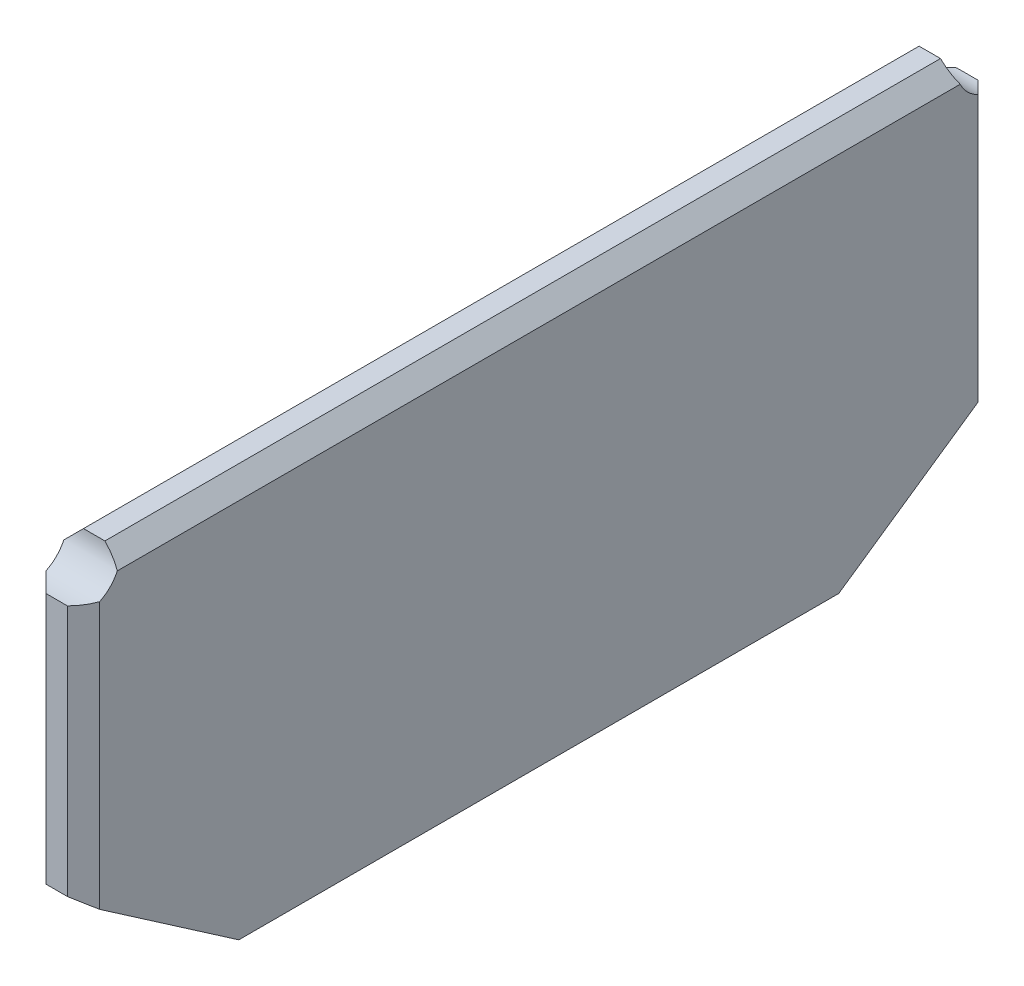
SolidWorks part; units mm, degrees
material "Q235-A"
ref_plane "Front Plane" through (0, 0, 0) normal (0, 0, 1) x (1, 0, 0)
ref_plane "Top Plane" through (0, 0, 0) normal (0, 1, 0) x (1, 0, 0)
ref_plane "Right Plane" through (0, 0, 0) normal (1, 0, 0) x (0, 0, -1)
sketch "Sketch1" plane through (0, 0, 0) normal (1, 0, 0) x (0, 0, -1)
  line L0 (0, 0) -> (0, 370) construction
  line L1 (-390, 370) -> (390, 370)
  line L2 (425, 335) -> (425, 100)
  line L3 (425, 100) -> (280, 0)
  line L4 (280, 0) -> (-280, 0)
  line L5 (-425, 100) -> (-280, 0)
  line L6 (-425, 335) -> (-425, 100)
  arc A0 (390, 370) -> (425, 335) centre (425, 370) ccw
  arc A1 (-390, 370) -> (-425, 335) centre (-425, 370) cw
  dimension "D2" = 35
  dimension "D1" = 850
  dimension "D3" = 145
  dimension "D4" = 100
  dimension "D5" = 370
extrude "Boss-Extrude1" add sketch "Sketch1" along normal mid plane 50
chamfer "Chamfer1" distance 15 angle 45 6 edges at (-25, 217.5, 425) (-25, 370, 0) (-25, 217.5, -425) (25, 217.5, -425) (25, 370, 0) (25, 217.5, 425)
